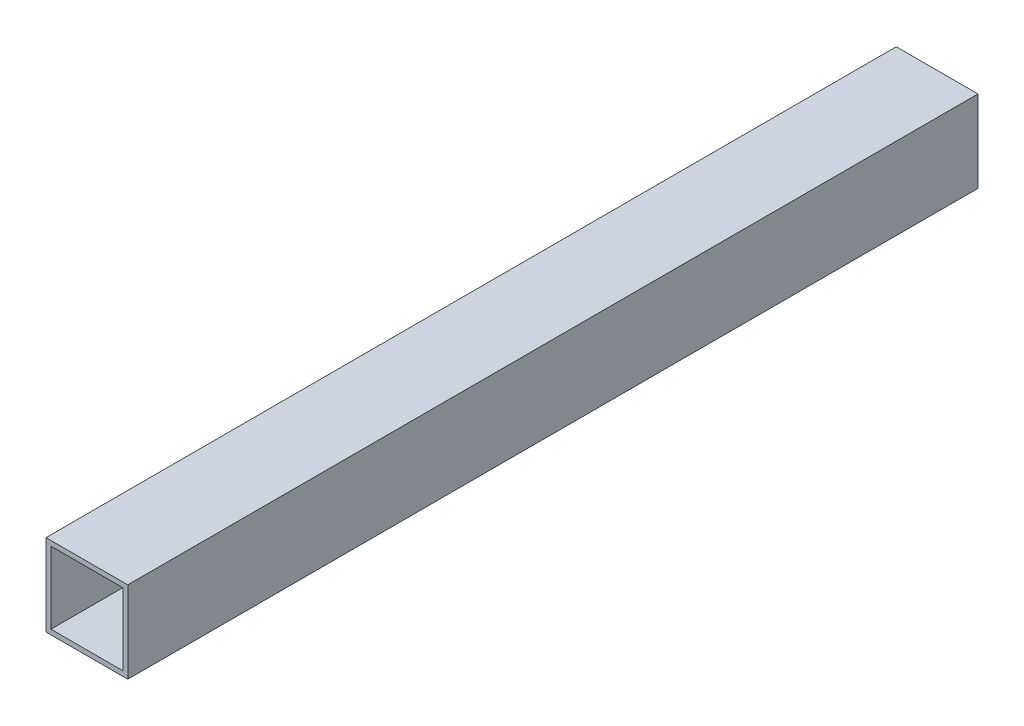
from build123d import *

# Parameters (mm, degrees)
SKETCH_1_W          = 50
SKETCH_1_H          = 50
SKETCH_1_W_2        = 44
SKETCH_1_H_2        = 44
EXTRUDE_1_DEPTH     = 520
SKETCH_2_W          = 56
SKETCH_2_H          = 56
CUT_EXTRUDE_1_DEPTH = 100
SKETCH_3_W          = 50
SKETCH_3_H          = 50
SKETCH_3_W_2        = 44
SKETCH_3_H_2        = 44
EXTRUDE_2_DEPTH     = 100


with BuildPart() as part:
    # 草图1 → 凸台-拉伸1 (new body)
    with BuildSketch(Plane.XY):
        with Locations((25, 25)):
            Rectangle(SKETCH_1_W, SKETCH_1_H)
        with Locations((25, 25)):
            Rectangle(SKETCH_1_W_2, SKETCH_1_H_2, mode=Mode.SUBTRACT)
    extrude(amount=EXTRUDE_1_DEPTH)

    # 草图2 → 切除-拉伸1 (cut)
    with BuildSketch(Plane.XY.offset(520)):
        with Locations((25, 25)):
            Rectangle(SKETCH_2_W, SKETCH_2_H)
    extrude(amount=-CUT_EXTRUDE_1_DEPTH, mode=Mode.SUBTRACT)

    # 草图3 → 凸台-拉伸2 (add)
    with BuildSketch(Plane.XY.offset(420)):
        with Locations((25, 25)):
            Rectangle(SKETCH_3_W, SKETCH_3_H)
        with Locations((25, 25)):
            Rectangle(SKETCH_3_W_2, SKETCH_3_H_2, mode=Mode.SUBTRACT)
    extrude(amount=EXTRUDE_2_DEPTH)


solid = part.part
